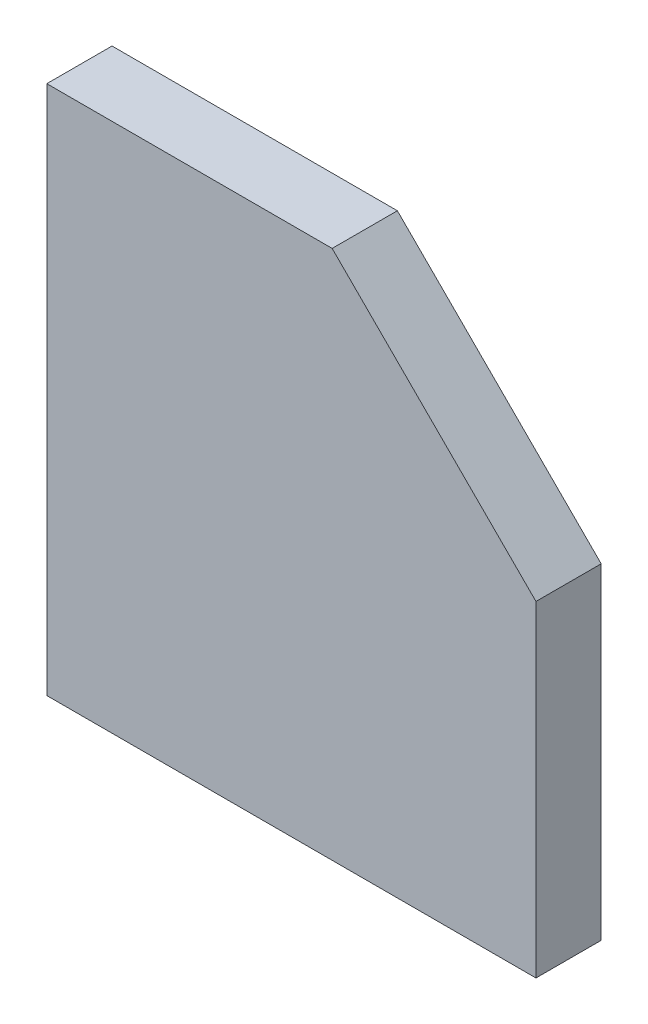
SolidWorks part; units mm, degrees
material "Q235"
ref_plane "Front Plane" through (0, 0, 0) normal (0, 0, 1) x (1, 0, 0)
ref_plane "Top Plane" through (0, 0, 0) normal (0, 1, 0) x (1, 0, 0)
ref_plane "Right Plane" through (0, 0, 0) normal (1, 0, 0) x (0, 0, -1)
sketch "Sketch1" plane through (0, 0, 0) normal (0, 0, 1) x (1, 0, 0)
  line L0 (0, 130) -> (0, 0)
  line L1 (0, 0) -> (120, 0)
  line L2 (120, 0) -> (120, 130)
  line L4 (120, 130) -> (0, 130)
  dimension "D1" = 120
  dimension "D2" = 130
extrude "Boss-Extrude1" add sketch "Sketch1" along normal mid plane 16
chamfer "Chamfer1" distance 50 angle 45 1 edges at (120, 130, 0)
